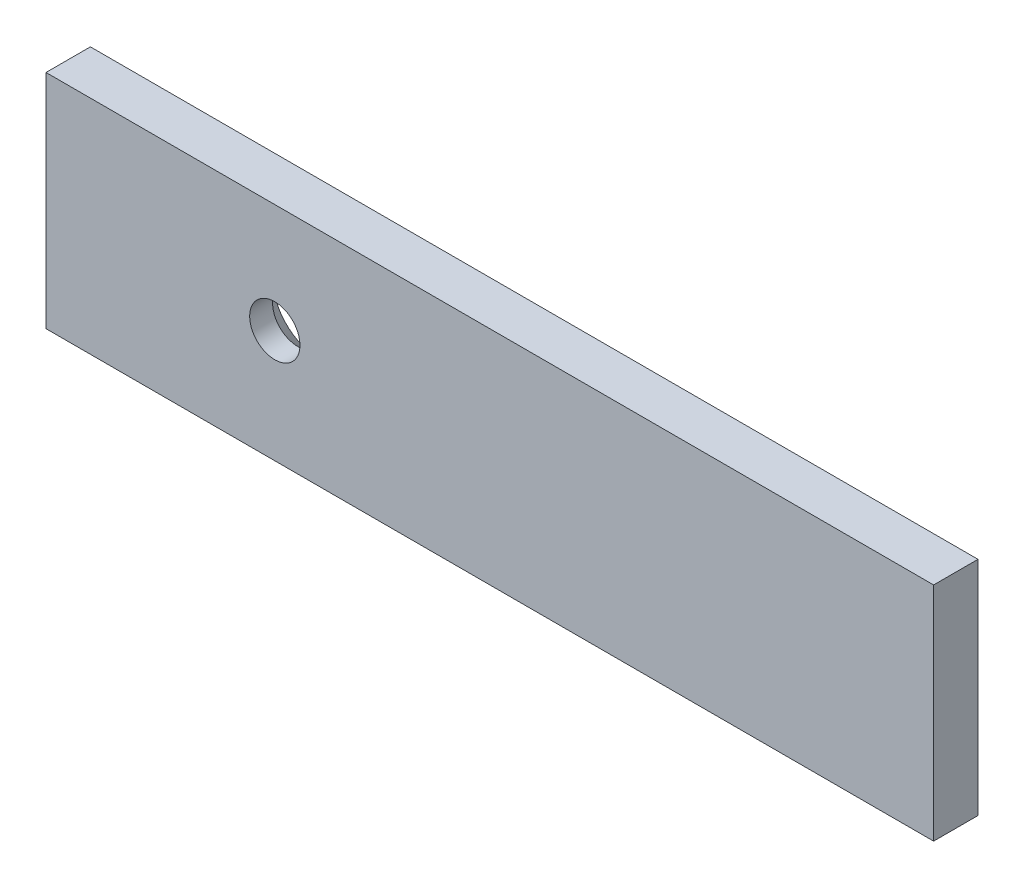
SolidWorks part; units mm, degrees
ref_plane "前视基准面" through (0, 0, 0) normal (0, 0, 1) x (1, 0, 0)
ref_plane "上视基准面" through (0, 0, 0) normal (0, 1, 0) x (1, 0, 0)
ref_plane "右视基准面" through (0, 0, 0) normal (1, 0, 0) x (0, 0, -1)
sketch "草图1" plane through (0, 0, 0) normal (0, 0, 1) x (1, 0, 0)
  line L1 (-30, -7.5) -> (30, -7.5)
  line L2 (-30, -7.5) -> (-30, 7.5)
  line L3 (-30, 7.5) -> (30, 7.5)
  line L4 (30, -7.5) -> (30, 7.5)
  line L5 (-30, -7.5) -> (30, 7.5) construction
  line L6 (-30, 7.5) -> (30, -7.5) construction
  point P0 (0, 0)
  dimension "D1" = 15
  dimension "D2" = 60
extrude "凸台-拉伸1" add sketch "草图1" along normal blind 3
hole_wizard "M3 十字切槽平头螺钉锥孔1" positions "3D草图2" profile "草图2" countersink size "M3" standard "IS" end condition up to next
sketch3d "3D草图2"
  point P0 (-14.5339, 0.1148, 0)
sketch "草图2" plane through (-14.5339, 0.1148, 0) normal (1, 0, 0) x (0, 1, 0)
  line L0 (0, 0) -> (0, 3)
  line L1 (0, 3) -> (1.7, 3)
  line L2 (1.7, 3) -> (1.7, 1.45)
  line L3 (1.7, 1.45) -> (3.15, 0)
  line L5 (3.15, 0) -> (0, 0)
  line L6 (-1.7, 1.45) -> (-3.15, 0) construction
  line L11 (0, -6.35) -> (0, 107.95) construction
  dimension "通孔孔直径" = 3.4
  dimension "通孔孔深度" = 3
  dimension "近端锥形沉头孔直径" = 6.3
  dimension "近端锥形沉头孔角度" = 90
